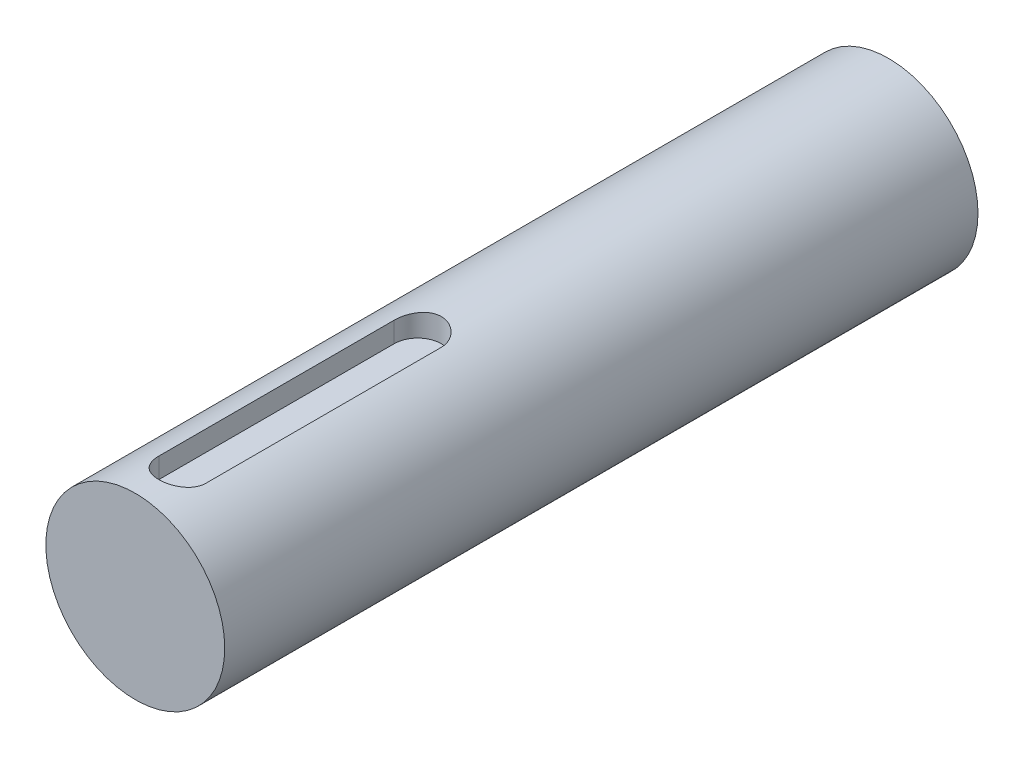
from build123d import *

# Parameters (mm, degrees)
SKETCH_1_R           = 19
BOSS_EXTRUDE_1_DEPTH = 160
CUT_EXTRUDE_1_DEPTH  = 165.468842034


with BuildPart() as part:
    # Sketch 1 → Boss-Extrude 1 (new body)
    with BuildSketch(Plane.XY):
        Circle(SKETCH_1_R)
    extrude(amount=BOSS_EXTRUDE_1_DEPTH)

    # Sketch 3 → Cut-Extrude 1 (cut, through all)
    with BuildSketch(Plane(origin=(0, 14, 0), x_dir=(1, 0, 0), z_dir=(0, 1, 0))):
        with BuildLine():
            Line((-5, -150), (-5, -100))
            ThreePointArc((-5, -100), (0, -95), (5, -100))
            Line((5, -100), (5, -150))
            ThreePointArc((5, -150), (0, -155), (-5, -150))
        make_face()
    extrude(amount=CUT_EXTRUDE_1_DEPTH, mode=Mode.SUBTRACT)


solid = part.part
